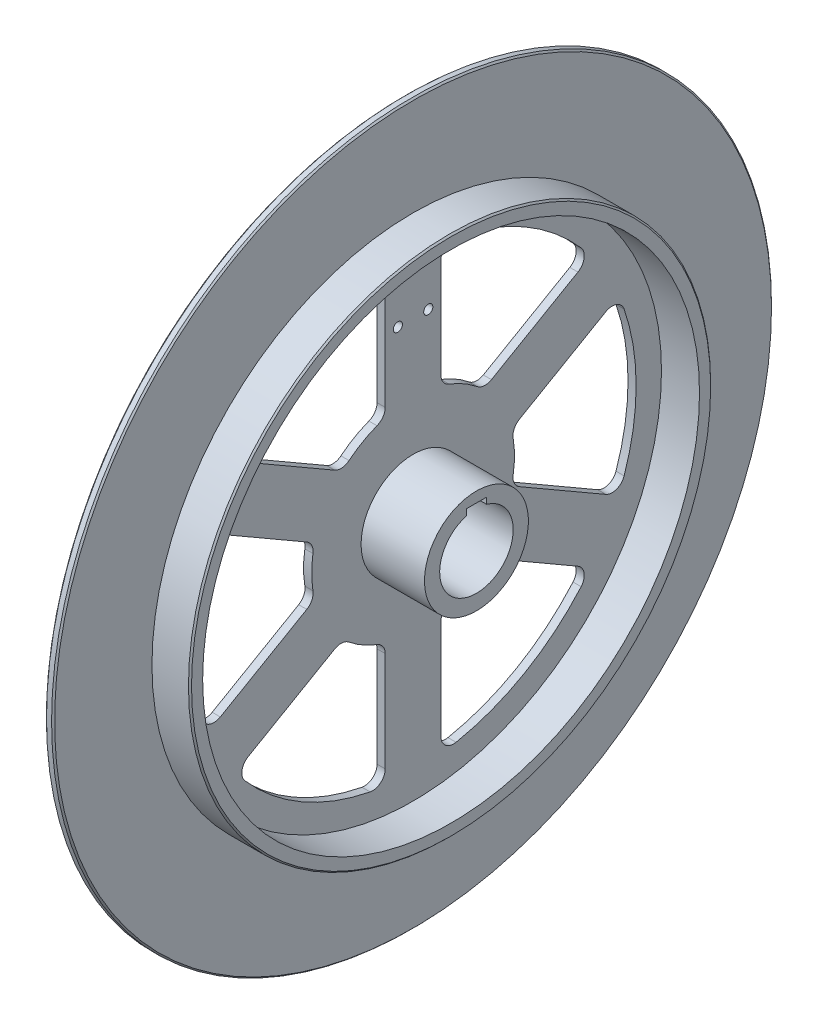
SolidWorks part; units mm, degrees
material "45"
ref_plane "Front Plane" through (0, 0, 0) normal (0, 0, 1) x (1, 0, 0)
ref_plane "Top Plane" through (0, 0, 0) normal (0, 1, 0) x (1, 0, 0)
ref_plane "Right Plane" through (0, 0, 0) normal (1, 0, 0) x (0, 0, -1)
sketch "Sketch1" plane through (0, 0, 0) normal (0, 0, 1) x (1, 0, 0)
  line L0 (-31, 550) -> (-31, 534)
  line L1 (109, 710) -> (125, 710)
  line L4 (79, 137.5) -> (79, 102.5)
  line L5 (125, 710) -> (125, 515)
  line L7 (109, 710) -> (109, 550)
  line L8 (-373.3517, 0) -> (373.3517, 0) construction
  line L9 (125, 490) -> (125, 102.5)
  line L10 (109, 534) -> (109, 137.5)
  line L11 (125, 102.5) -> (250, 102.5)
  line L12 (79, 137.5) -> (109, 137.5)
  line L13 (-31, 550) -> (109, 550)
  line L14 (-31, 534) -> (109, 534)
  line L15 (125, 515) -> (200, 515)
  line L16 (125, 490) -> (200, 490)
  line L17 (0, 102.5) -> (79, 102.5)
  line L18 (0, 72.5) -> (250, 72.5)
  line L19 (125, 102.5) -> (250, 102.5)
  line L20 (200, 515) -> (200, 490)
  line L21 (250, 102.5) -> (250, 72.5)
  line L22 (0, 102.5) -> (0, 72.5)
  dimension "D1" = 125
  dimension "D2" = 16
  dimension "D3" = 1030
  dimension "D4" = 25
  dimension "D5" = 1420
  dimension "D6" = 1100
  dimension "D7" = 140
  dimension "D8" = 275
  dimension "D9" = 30
  dimension "D10" = 250
  dimension "D11" = 145
  dimension "D12" = 30
  dimension "D13" = 75
  dimension "D14" = 16
revolve "Revolve1" add sketch "Sketch1" angle 360 about L8
sketch "Sketch3" plane through (109, 0, 0) normal (-1, 0, 0) x (0, 0, 1)
  line L0 (-55, 407.2162) -> (-55, 210.2974)
  line L1 (-154.6229, 152.7801) -> (-325.1595, 251.2395)
  line L2 (0, 0) -> (0, 655.2261) construction
  arc A0 (-71.1111, 186.931) -> (-126.3315, 155.0495) centre (0, 0) ccw
  arc A1 (-331.4945, 289.3293) -> (-84.8193, 431.7473) centre (0, 0) cw
  circle A2 centre (0, 0) radius 534 construction
  arc A3 (-55, 210.2974) -> (-71.1111, 186.931) centre (-80, 210.2974) cw
  arc A4 (-126.3315, 155.0495) -> (-154.6229, 152.7801) centre (-142.1229, 174.4307) cw
  arc A5 (-55, 407.2162) -> (-84.8193, 431.7473) centre (-80, 407.2162) ccw
  arc A6 (-325.1595, 251.2395) -> (-331.4945, 289.3293) centre (-312.6595, 272.8901) cw
  dimension "D1" = 200
  dimension "D2" = 440
  dimension "D5" = 25
  dimension "D3" = 110
  dimension "D4" = 60
extrude "Cut-Extrude1" cut sketch "Sketch3" against normal through all
pattern_circular "CirPattern1" count 6 over 360 about axis through (0, 0, 0) along (1, 0, 0) of "Cut-Extrude1"
sketch "Sketch4" plane through (109, 0, 0) normal (-1, 0, 0) x (0, 0, 1)
  line L0 (-8, 533.9401) -> (-8, 102.1873)
  line L1 (8, 533.9401) -> (8, 102.1873)
  line L2 (0, 0) -> (0, 614.7598) construction
  circle A1 centre (0, 0) radius 102.5 construction
  circle A3 centre (0, 0) radius 102.5 construction
  circle A4 centre (0, 0) radius 534 construction
  circle A5 centre (0, 0) radius 534 construction
  arc A6 (8, 533.9401) -> (-8, 533.9401) centre (0, 0) ccw
  arc A7 (8, 102.1873) -> (-8, 102.1873) centre (0, 0) ccw
  dimension "D1" = 16
extrude "Boss-Extrude1" add sketch "Sketch4" along normal up to surface (109 mm away) up to face at (0, 0, 72.5)
fillet "Fillet2" radius 10 8 edges at (109, 335.6036, -8) (94, 137.2671, -8) (39.5, 102.1873, -8) (39.5, 102.1873, 8) (94, 137.2671, 8) (109, 335.6036, 8) (54.5, 533.9401, 8) (54.5, 533.9401, -8)
pattern_circular "CirPattern2" count 6 over 360 about axis through (0, 0, 0) along (1, 0, 0) of "Boss-Extrude1", "Fillet2"
sketch "Sketch5" plane through (109, 0, 0) normal (-1, 0, 0) x (0, 0, 1)
  line L1 (-30, 425) -> (30, 425) construction
  line L2 (-30, 425) -> (-30, 335) construction
  line L3 (-30, 335) -> (30, 335) construction
  line L4 (30, 425) -> (30, 335) construction
  line L5 (-30, 425) -> (30, 335) construction
  line L6 (-30, 335) -> (30, 425) construction
  circle A0 centre (-30, 425) radius 9
  circle A1 centre (-30, 335) radius 9
  circle A2 centre (30, 335) radius 9
  circle A3 centre (30, 425) radius 9
  point P0 (0, 380)
  dimension "D3" = 18
  dimension "D1" = 60
  dimension "D2" = 90
  dimension "D4" = 380
extrude "Cut-Extrude2" cut sketch "Sketch5" against normal through all
sketch "Sketch6" plane through (0, 0, 8) normal (0, 0, 1) x (1, 0, 0)
  line L0 (109, 533.6907) -> (109, 136.3167) construction
  line L1 (94, 380) -> (40.8749, 380) construction
  line L2 (94, 395) -> (109, 395)
  line L3 (109, 395) -> (109, 365)
  line L4 (109, 365) -> (94, 365)
  arc A0 (94, 395) -> (94, 365) centre (94, 380) ccw
  dimension "D1" = 30
extrude "Cut-Extrude3" cut sketch "Sketch6" against normal through all and the other way blind 20
chamfer "Chamfer1" distance 3 angle 45 4 edges at (200, 0, 515) (125, 0, 710) (-31, 0, 550) (109, 0, 710)
sketch "Sketch7" plane through (0, 0, 0) normal (-1, 0, 0) x (0, 0, 1)
  line L1 (-20, 81.9) -> (20, 81.9)
  line L2 (-20, 81.9) -> (-20, 63.1)
  line L3 (-20, 63.1) -> (20, 63.1)
  line L4 (20, 81.9) -> (20, 63.1)
  line L5 (-20, 81.9) -> (20, 63.1) construction
  line L6 (-20, 63.1) -> (20, 81.9) construction
  circle A0 centre (0, 0) radius 72.5 construction
  point P0 (0, 72.5)
  dimension "D1" = 40
  dimension "D2" = 9.4
extrude "Cut-Extrude4" cut sketch "Sketch7" against normal through all
sketch "Sketch8" plane through (0, 0, 0) normal (0, 0, 1) x (1, 0, 0)
  line L0 (109, 550) -> (-31, 550)
  line L1 (-31, 550) -> (-31, 146.3976)
  line L2 (79, 136.4723) -> (109, 136.4723)
  line L4 (109, 707) -> (109, -707) construction
  line L5 (-31, 547) -> (-31, -547) construction
  line L6 (79, 136.4723) -> (79, 101.1795)
  line L7 (79, 146.3976) -> (79, 136.4723) construction
  line L8 (79, 136.4723) -> (79, 82.7678) construction
  line L9 (79, 101.1795) -> (49, 101.1795)
  line L10 (49, 101.1795) -> (49, 0)
  line L11 (49, 0) -> (-31, 0)
  line L12 (-31, 0) -> (-31, 146.3976)
  line L13 (79, 101.1795) -> (0, 101.1795) construction
  line L14 (109, 136.4723) -> (109, 550)
  line L15 (0, 0) -> (-281.5361, 0) construction
  line L16 (108.9253, 136.4723) -> (79, 136.4723) construction
  dimension "D1" = 30
revolve "Cut-Revolve1" cut sketch "Sketch8" angle 360 about L15
